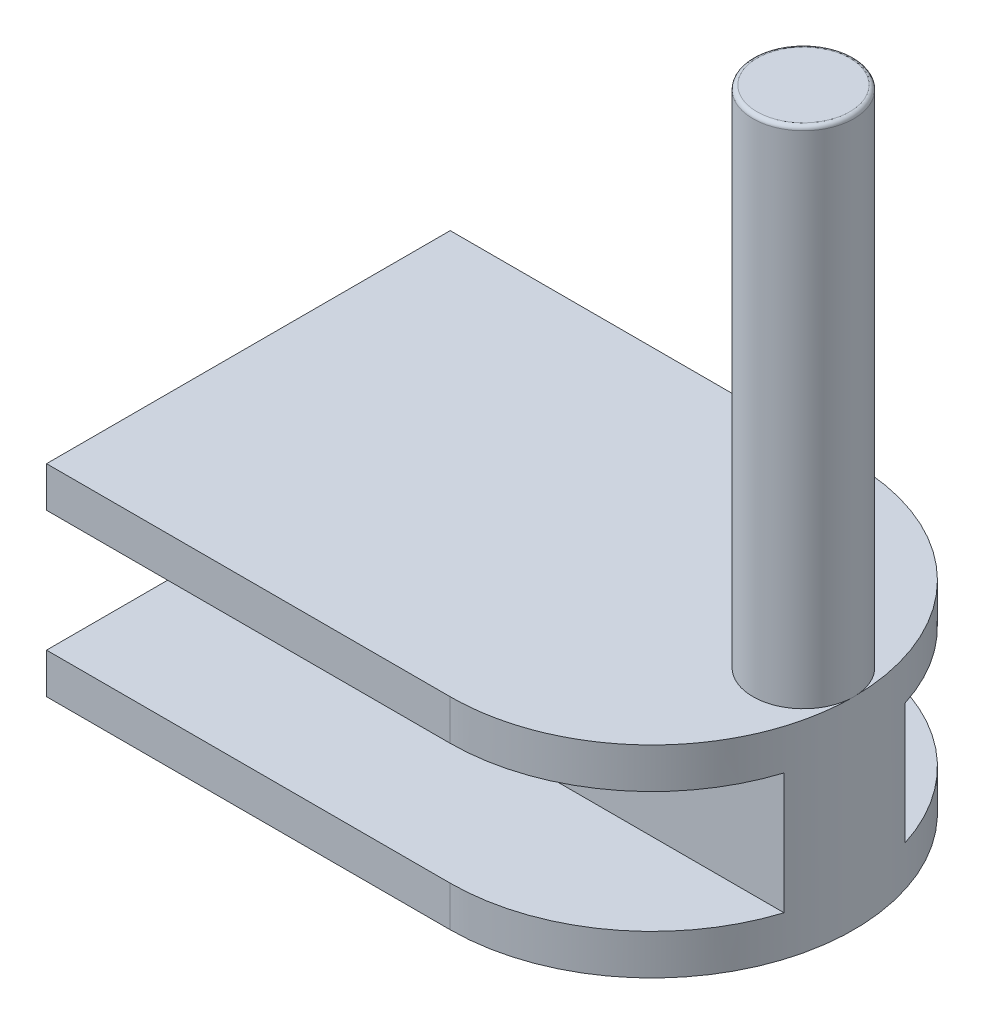
SolidWorks part; units mm, degrees
ref_plane "Front Plane" through (0, 0, 0) normal (0, 0, 1) x (1, 0, 0)
ref_plane "Top Plane" through (0, 0, 0) normal (0, 1, 0) x (1, 0, 0)
ref_plane "Right Plane" through (0, 0, 0) normal (1, 0, 0) x (0, 0, -1)
sketch "Sketch1" plane through (0, 0, 0) normal (0, 1, 0) x (1, 0, 0)
  line L1 (0, 0) -> (30, 0)
  line L2 (0, 0) -> (0, 20)
  line L3 (0, 20) -> (30, 20)
  line L4 (30, 0) -> (30, 20)
  dimension "D1" = 20
  dimension "D2" = 30
extrude "Boss-Extrude1" add sketch "Sketch1" along normal blind 10
sketch "Sketch2" plane through (0, 0, 0) normal (-1, 0, 0) x (0, 0, 1)
  line L0 (-20, 5) -> (0, 5) construction
  line L1 (-20, 10) -> (-20, 0) construction
  line L2 (0, 10) -> (0, 0) construction
  line L3 (-20, 10) -> (0, 10) construction
  line L4 (-20, 8) -> (-13, 8)
  line L5 (-20, 8) -> (-20, 2)
  line L6 (-20, 2) -> (-13, 2)
  line L7 (0, 8) -> (0, 2)
  line L8 (-20, 0) -> (0, 0) construction
  line L9 (-13, 8) -> (-13, 2)
  line L10 (-7, 8) -> (-7, 2)
  line L11 (-7, 8) -> (0, 8)
  line L12 (-7, 2) -> (0, 2)
  dimension "D1" = 2
  dimension "D2" = 2
  dimension "D3" = 7
  dimension "D4" = 7
extrude "Cut-Extrude1" cut sketch "Sketch2" against normal through all
sketch "Sketch3" plane through (0, 10, 0) normal (0, 1, 0) x (1, 0, 0)
  line L0 (30, 20) -> (0, 20) construction
  line L1 (0, 0) -> (30, 0) construction
  line L2 (30, 10) -> (0, 10) construction
  line L3 (0, 20) -> (0, 0) construction
  line L4 (30, 0) -> (30, 20) construction
  line L5 (30, 20) -> (20, 20)
  line L6 (30, 0) -> (30, 20)
  line L7 (20, 0) -> (30, 0)
  arc A0 (20, 20) -> (20, 0) centre (20, 10) cw
  line M2 (0, 0) -> (30, 0)
  line M3 (30, 0) -> (30, 20)
  line M4 (30, 20) -> (0, 20)
  dimension "D1" = 10
extrude "Cut-Extrude2" cut sketch "Sketch3" against normal through all contours A0 M3 M2 | A0 L6 M4
sketch "Sketch4" plane through (0, 10, 0) normal (0, 1, 0) x (1, 0, 0)
  line L0 (30, 10) -> (0, 10) construction
  line L1 (0, 20) -> (0, 0) construction
  arc A0 (20, 0) -> (20, 20) centre (20, 10) ccw construction
  circle A1 centre (27.5, 10) radius 2.5
  dimension "D1" = 5
extrude "Boss-Extrude2" add sketch "Sketch4" along normal blind 25
fillet "Fillet1" radius 0.2 1 edges at (27.5, 35, -7.5)
